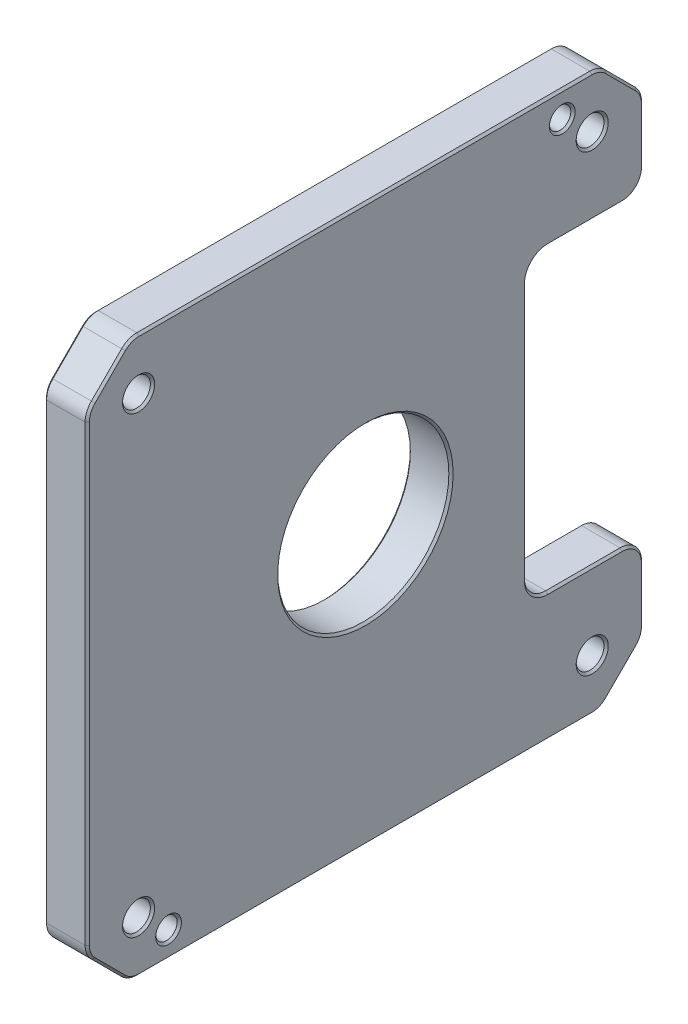
from build123d import *

# Parameters (mm, degrees)
SKETCH_1_W          = 130
SKETCH_1_H          = 130
EXTRUDE_1_DEPTH     = 10
SKETCH_2_W          = 60
SKETCH_2_H          = 70
CUT_EXTRUDE_1_DEPTH = 93.466210045
CHAMFER_1_SIZE      = 10
SKETCH_3_R          = 3.25
CUT_EXTRUDE_2_DEPTH = 93.466210045
SKETCH_4_R          = 2.5
CUT_EXTRUDE_3_DEPTH = 93.466210045
SKETCH_5_R          = 20
CUT_EXTRUDE_6_DEPTH = 93.466210045
FILLET_1_R          = 5
FILLET_2_R          = 5
CHAMFER_2_SIZE      = 0.5


with BuildPart() as part:
    # 草图1 → 凸台-拉伸1 (new body)
    with BuildSketch(Plane(origin=(0, 0, 0), x_dir=(0, 0, -1), z_dir=(1, 0, 0))):
        Rectangle(SKETCH_1_W, SKETCH_1_H)
    extrude(amount=EXTRUDE_1_DEPTH)

    # 草图2 → 切除-拉伸1 (cut, through all)
    with BuildSketch(Plane(origin=(10, 0, 0), x_dir=(0, 0, -1), z_dir=(1, 0, 0))):
        with Locations((67.64, 0)):
            Rectangle(SKETCH_2_W, SKETCH_2_H)
    extrude(amount=-CUT_EXTRUDE_1_DEPTH, mode=Mode.SUBTRACT)

    # 倒角1
    chamfer_1_edges = [part.edges().sort_by_distance(p)[0] for p in [
        (5, -65, -65),
        (5, -65, 65),
        (5, 65, 65),
        (5, 65, -65),
    ]]
    chamfer(chamfer_1_edges, length=CHAMFER_1_SIZE)

    # 草图3 → 切除-拉伸2 (cut, through all)
    with BuildSketch(Plane(origin=(10, 0, 0), x_dir=(0, 0, -1), z_dir=(1, 0, 0))):
        with Locations((-53, -53)):
            Circle(SKETCH_3_R)
        with Locations((-53, 53)):
            Circle(SKETCH_3_R)
        with Locations((53, -53)):
            Circle(SKETCH_3_R)
        with Locations((53, 53)):
            Circle(SKETCH_3_R)
    extrude(amount=-CUT_EXTRUDE_2_DEPTH, mode=Mode.SUBTRACT)

    # 草图4 → 切除-拉伸3 (cut, through all)
    with BuildSketch(Plane(origin=(10, 0, 0), x_dir=(0, 0, -1), z_dir=(1, 0, 0))):
        with Locations((-46, -59)):
            Circle(SKETCH_4_R)
        with Locations((46, 59)):
            Circle(SKETCH_4_R)
    extrude(amount=-CUT_EXTRUDE_3_DEPTH, mode=Mode.SUBTRACT)

    # 草图5 → 切除-拉伸6 (cut, through all)
    with BuildSketch(Plane.ZY):
        Circle(SKETCH_5_R)
    extrude(amount=-CUT_EXTRUDE_6_DEPTH, mode=Mode.SUBTRACT)

    # 圆角1
    fillet_1_edges = [part.edges().sort_by_distance(p)[0] for p in [
        (5, 35, -37.64),
        (5, -35, -37.64),
    ]]
    fillet(fillet_1_edges, radius=FILLET_1_R)

    # 圆角2
    fillet_2_edges = [part.edges().sort_by_distance(p)[0] for p in [
        (5, -35, -65),
        (5, 35, -65),
        (5, 65, 55),
        (5, 65, -55),
        (5, 55, -65),
        (5, -55, -65),
        (5, -65, 55),
        (5, -65, -55),
        (5, -55, 65),
        (5, 55, 65),
    ]]
    fillet(fillet_2_edges, radius=FILLET_2_R)

    # 倒角2
    chamfer_2_edges = [part.edges().sort_by_distance(p)[0] for p in [
        (10, 65, 0),
        (0, 65, 0),
        (10, 46.464466094, -65),
        (10, 60, -60),
        (10, 60, 60),
        (10, 0, 65),
        (10, -60, 60),
        (10, -65, 0),
        (10, -60, -60),
        (10, -46.464466094, -65),
        (10, 35, -51.32),
        (10, -64.619397663, 54.84234935),
        (10, -54.84234935, 64.619397663),
        (10, 64.619397663, -54.84234935),
        (10, 54.84234935, -64.619397663),
        (10, 36.464466094, -63.535533906),
        (10, -36.464466094, -63.535533906),
        (10, -54.84234935, -64.619397663),
        (10, -64.619397663, -54.84234935),
        (10, 54.84234935, 64.619397663),
        (10, 64.619397663, 54.84234935),
        (0, 60, 60),
        (0, 60, -60),
        (0, 46.464466094, -65),
        (0, 35, -51.32),
        (0, -46.464466094, -65),
        (0, -60, -60),
        (0, -65, 0),
        (0, -60, 60),
        (0, 0, 65),
        (0, -64.619397663, 54.84234935),
        (0, -54.84234935, 64.619397663),
        (0, 64.619397663, -54.84234935),
        (0, 54.84234935, -64.619397663),
        (0, 36.464466094, -63.535533906),
        (0, -36.464466094, -63.535533906),
        (0, -54.84234935, -64.619397663),
        (0, -64.619397663, -54.84234935),
        (0, 54.84234935, 64.619397663),
        (0, 64.619397663, 54.84234935),
        (0, -53, 56.25),
        (10, -53, 56.25),
        (0, 53, 56.25),
        (10, 53, 56.25),
        (0, -53, -49.75),
        (10, -53, -49.75),
        (0, 53, -49.75),
        (10, 53, -49.75),
        (0, -59, 48.5),
        (10, -59, 48.5),
        (0, 59, -43.5),
        (10, 59, -43.5),
        (10, 0, -20),
        (0, 0, -20),
        (0, -35, -51.32),
        (10, -35, -51.32),
        (10, 0, -37.64),
        (0, 0, -37.64),
        (10, -33.535533906, -39.104466094),
        (0, -33.535533906, -39.104466094),
        (10, 33.535533906, -39.104466094),
        (0, 33.535533906, -39.104466094),
    ]]
    chamfer(chamfer_2_edges, length=CHAMFER_2_SIZE)


solid = part.part
